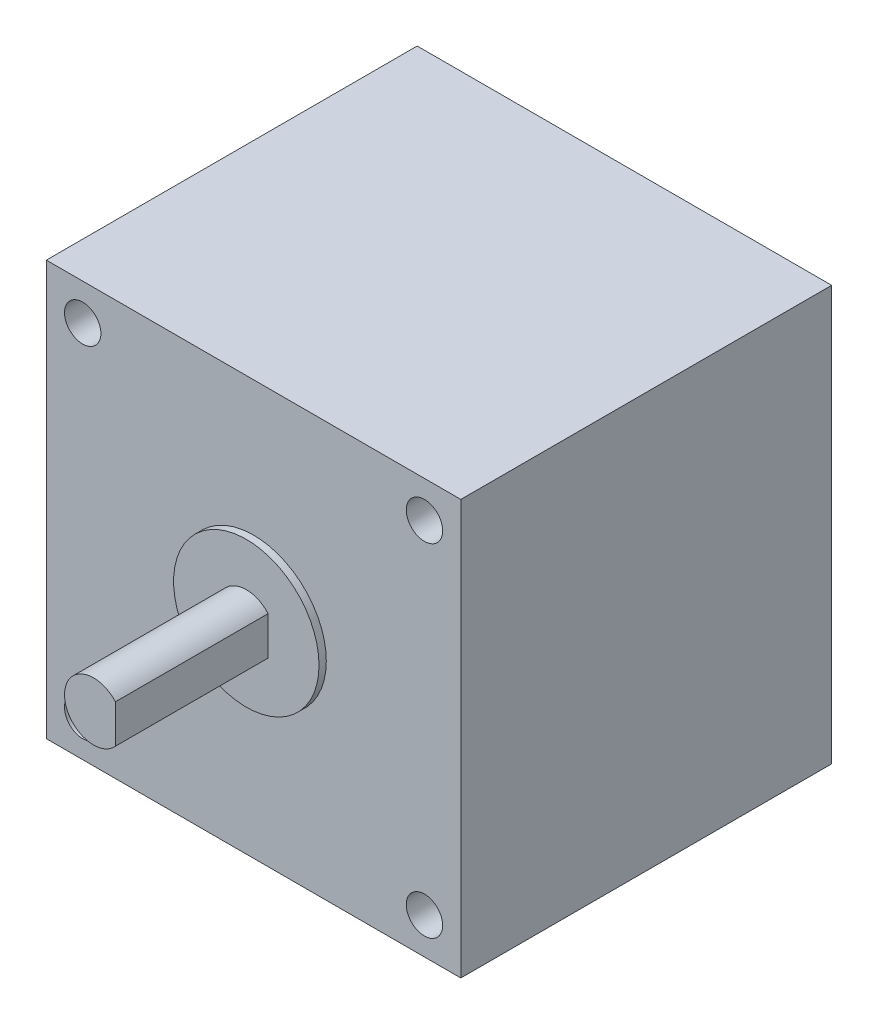
SolidWorks part; units mm, degrees
ref_plane "Front Plane" through (0, 0, 0) normal (0, 0, 1) x (1, 0, 0)
ref_plane "Top Plane" through (0, 0, 0) normal (0, 1, 0) x (1, 0, 0)
ref_plane "Right Plane" through (0, 0, 0) normal (1, 0, 0) x (0, 0, -1)
sketch "Sketch1" plane through (0, 0, 0) normal (0, 0, 1) x (1, 0, 0)
  line L1 (28.5, -28.5) -> (-28.5, -28.5)
  line L2 (28.5, -28.5) -> (28.5, 28.5)
  line L3 (28.5, 28.5) -> (-28.5, 28.5)
  line L4 (-28.5, -28.5) -> (-28.5, 28.5)
  line L5 (28.5, -28.5) -> (-28.5, 28.5) construction
  line L6 (28.5, 28.5) -> (-28.5, -28.5) construction
  point P0 (0, 0)
  dimension "D1" = 57
extrude "Boss-Extrude1" add sketch "Sketch1" along normal blind 51
sketch "Sketch2" plane through (0, 0, 51) normal (0, 0, 1) x (1, 0, 0)
  line L1 (23.5, -23.5) -> (-23.5, -23.5) construction
  line L2 (23.5, -23.5) -> (23.5, 23.5) construction
  line L3 (23.5, 23.5) -> (-23.5, 23.5) construction
  line L4 (-23.5, -23.5) -> (-23.5, 23.5) construction
  line L5 (23.5, -23.5) -> (-23.5, 23.5) construction
  line L6 (23.5, 23.5) -> (-23.5, -23.5) construction
  circle A0 centre (-23.5, 23.5) radius 2.5
  circle A1 centre (23.5, 23.5) radius 2.5
  circle A2 centre (23.5, -23.5) radius 2.5
  circle A3 centre (-23.5, -23.5) radius 2.5
  point P0 (0, 0)
  dimension "D1" = 5
  dimension "D2" = 47
extrude "Cut-Extrude1" cut sketch "Sketch2" against normal blind 98
sketch "Sketch4" plane through (0, 0, 51) normal (0, 0, 1) x (1, 0, 0)
  circle A0 centre (0, 0) radius 10
  dimension "D1" = 20
extrude "Boss-Extrude2" add sketch "Sketch4" along normal blind 1
sketch "Sketch5" plane through (0, 0, 52) normal (0, 0, 1) x (1, 0, 0)
  circle A0 centre (0, 0) radius 4
  dimension "D1" = 8
extrude "Boss-Extrude3" add sketch "Sketch5" along normal blind 21
sketch "Sketch6" plane through (0, 0, 73) normal (0, 0, 1) x (1, 0, 0)
  line L0 (3, 2.6458) -> (3, -2.6458)
  circle A0 centre (0, 0) radius 4 construction
  circle A1 centre (0, 0) radius 4
  circle M2 centre (0, 0) radius 4
  dimension "D1" = 3
extrude "Cut-Extrude2" cut sketch "Sketch6" against normal blind 21 contours L0 M2
